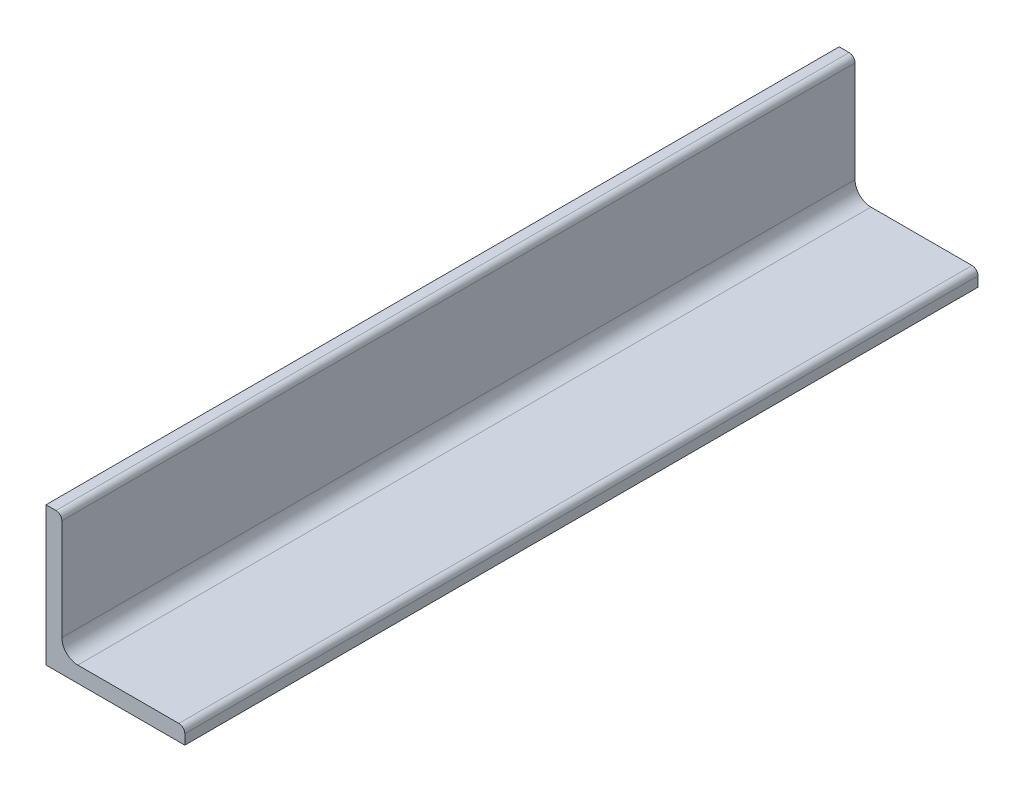
from build123d import *

# Parameters (mm, degrees)
BOSS_EXTRUDE1_DEPTH = 400


with BuildPart() as part:
    # Sketch1 → Boss-Extrude1 (new body)
    with BuildSketch(Plane.XY):
        with BuildLine():
            Line((0, 70), (0, 0))
            Line((0, 0), (70, 0))
            Line((70, 0), (70, 5))
            ThreePointArc((70, 5), (69.121320344, 7.121320344), (67, 8))
            Line((67, 8), (16, 8))
            ThreePointArc((16, 8), (10.343145751, 10.343145751), (8, 16))
            Line((8, 16), (8, 67))
            ThreePointArc((8, 67), (7.121320344, 69.121320344), (5, 70))
            Line((5, 70), (0, 70))
        make_face()
    extrude(amount=BOSS_EXTRUDE1_DEPTH)


solid = part.part
